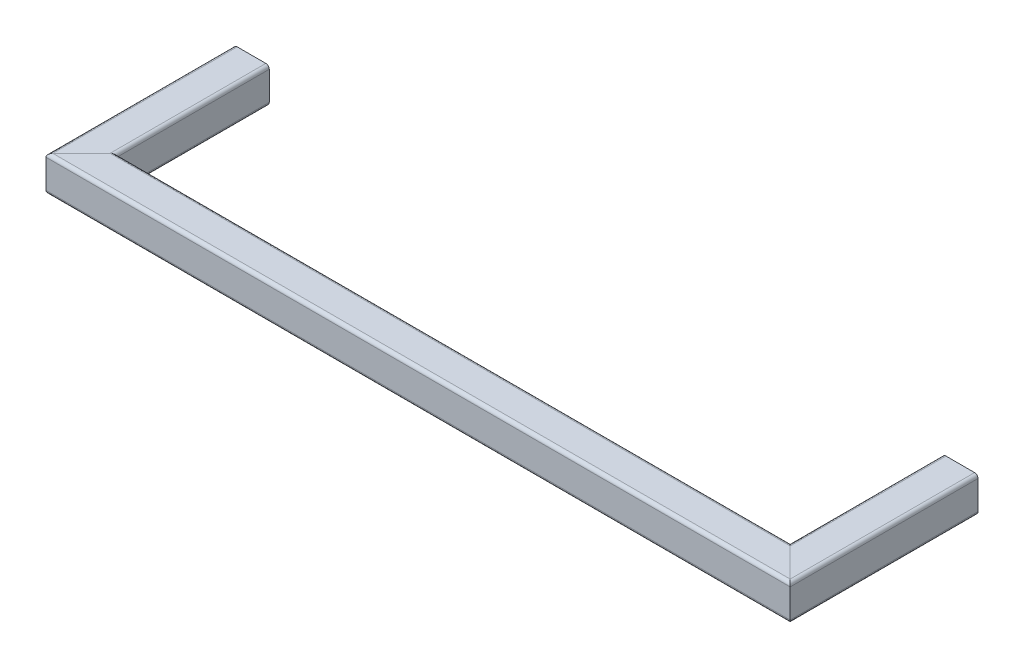
SolidWorks part; units mm, degrees
ref_plane "Front Plane" through (0, 0, 0) normal (0, 0, 1) x (1, 0, 0)
ref_plane "Top Plane" through (0, 0, 0) normal (0, 1, 0) x (1, 0, 0)
ref_plane "Right Plane" through (0, 0, 0) normal (1, 0, 0) x (0, 0, -1)
sketch "Sketch1" plane through (0, 0, 0) normal (0, 1, 0) x (1, 0, 0)
  line L0 (-250, 0) -> (250, 0)
  line L1 (-250, 0) -> (-250, 120)
  line L2 (0, 0) -> (0, 66.6058) construction
  line L3 (250, 0) -> (250, 120)
  point P4 (0, 0)
  dimension "D1" = 500
  dimension "D2" = 120
other "Gb／6728-1986 square hollow section 025 X 25 X 1.2(1)"
ref_plane "Plane1" through (-250, 0, 0) normal (0, 0, -1) x (-1, 0, 0)
sketch "Sketch11" plane through (-250, 0, 0) normal (0, 0, -1) x (-1, 0, 0)
  line L0 (-10.1, -11.3) -> (10.1, -11.3)
  line L1 (-11.3, -10.1) -> (-11.3, 10.1)
  line L2 (10.1, 11.3) -> (-10.1, 11.3)
  line L3 (11.3, 10.1) -> (11.3, -10.1)
  line L4 (-10.1, -12.5) -> (10.1, -12.5)
  line L5 (-12.5, -10.1) -> (-12.5, 10.1)
  line L6 (10.1, 12.5) -> (-10.1, 12.5)
  line L7 (12.5, 10.1) -> (12.5, -10.1)
  arc A0 (12.5, 10.1) -> (10.1, 12.5) centre (10.1, 10.1) ccw
  arc A1 (10.1, -12.5) -> (12.5, -10.1) centre (10.1, -10.1) ccw
  arc A2 (-12.5, -10.1) -> (-10.1, -12.5) centre (-10.1, -10.1) ccw
  arc A3 (-10.1, 12.5) -> (-12.5, 10.1) centre (-10.1, 10.1) ccw
  arc A4 (-10.1, 11.3) -> (-11.3, 10.1) centre (-10.1, 10.1) ccw
  arc A5 (11.3, 10.1) -> (10.1, 11.3) centre (10.1, 10.1) ccw
  arc A6 (10.1, -11.3) -> (11.3, -10.1) centre (10.1, -10.1) ccw
  arc A7 (-11.3, -10.1) -> (-10.1, -11.3) centre (-10.1, -10.1) ccw
  point P0 (-12.5, 0)
  point P1 (12.5, 0)
  point P2 (0, 12.5)
  point P3 (0, -12.5)
  point P4 (0, 0)
  point P5 (-12.5, -12.5)
  point P6 (12.5, -12.5)
  point P7 (12.5, 12.5)
  point P8 (-12.5, 12.5)
  point P33 (0, 0)
  dimension "D1" = 2.4
  dimension "Thickness" = 1.2
  dimension "V_leg" = 25
sketch "Sketch2" plane through (0, 0, -120) normal (0, 0, -1) x (-1, 0, 0)
  line L4 (-262.5, 10.1) -> (-262.5, -10.1)
  line L5 (-260.1, -12.5) -> (-239.9, -12.5)
  line L6 (-237.5, -10.1) -> (-237.5, 10.1)
  line L7 (-239.9, 12.5) -> (-260.1, 12.5)
  line L8 (-262.5, 10.1) -> (-262.5, -10.1)
  line L9 (-260.1, -12.5) -> (-239.9, -12.5)
  line L10 (-237.5, -10.1) -> (-237.5, 10.1)
  line L11 (-239.9, 12.5) -> (-260.1, 12.5)
  line L12 (260.1, 12.5) -> (239.9, 12.5)
  line L13 (237.5, 10.1) -> (237.5, -10.1)
  line L14 (239.9, -12.5) -> (260.1, -12.5)
  line L15 (262.5, -10.1) -> (262.5, 10.1)
  line L16 (260.1, 12.5) -> (239.9, 12.5)
  line L17 (237.5, 10.1) -> (237.5, -10.1)
  line L18 (239.9, -12.5) -> (260.1, -12.5)
  line L19 (262.5, -10.1) -> (262.5, 10.1)
  arc A4 (-260.1, 12.5) -> (-262.5, 10.1) centre (-260.1, 10.1) ccw
  arc A5 (-262.5, -10.1) -> (-260.1, -12.5) centre (-260.1, -10.1) ccw
  arc A6 (-239.9, -12.5) -> (-237.5, -10.1) centre (-239.9, -10.1) ccw
  arc A7 (-237.5, 10.1) -> (-239.9, 12.5) centre (-239.9, 10.1) ccw
  arc A8 (-260.1, 12.5) -> (-262.5, 10.1) centre (-260.1, 10.1) ccw
  arc A9 (-262.5, -10.1) -> (-260.1, -12.5) centre (-260.1, -10.1) ccw
  arc A10 (-239.9, -12.5) -> (-237.5, -10.1) centre (-239.9, -10.1) ccw
  arc A11 (-237.5, 10.1) -> (-239.9, 12.5) centre (-239.9, 10.1) ccw
  arc A12 (262.5, 10.1) -> (260.1, 12.5) centre (260.1, 10.1) ccw
  arc A13 (239.9, 12.5) -> (237.5, 10.1) centre (239.9, 10.1) ccw
  arc A14 (237.5, -10.1) -> (239.9, -12.5) centre (239.9, -10.1) ccw
  arc A15 (260.1, -12.5) -> (262.5, -10.1) centre (260.1, -10.1) ccw
  arc A16 (262.5, 10.1) -> (260.1, 12.5) centre (260.1, 10.1) ccw
  arc A17 (239.9, 12.5) -> (237.5, 10.1) centre (239.9, 10.1) ccw
  arc A18 (237.5, -10.1) -> (239.9, -12.5) centre (239.9, -10.1) ccw
  arc A19 (260.1, -12.5) -> (262.5, -10.1) centre (260.1, -10.1) ccw
  dimension "D1" = 0
  dimension "D2" = 0
extrude "Boss-Extrude1" add sketch "Sketch2" against normal blind 3
sketch "Sketch3" plane through (0, -12.5, 0) normal (0, -1, 0) x (1, 0, 0)
  line L0 (250, -120) -> (250, -105) construction
  line L1 (239.9, -120) -> (260.1, -120) construction
  line L2 (0, 0) -> (0, -111.6676) construction
  line L3 (-250, -120) -> (-250, -105) construction
  circle A0 centre (250, -105) radius 5
  circle A1 centre (-250, -105) radius 5
  dimension "D1" = 10
  dimension "D2" = 15
extrude "Cut-Extrude1" cut sketch "Sketch3" against normal blind 2
